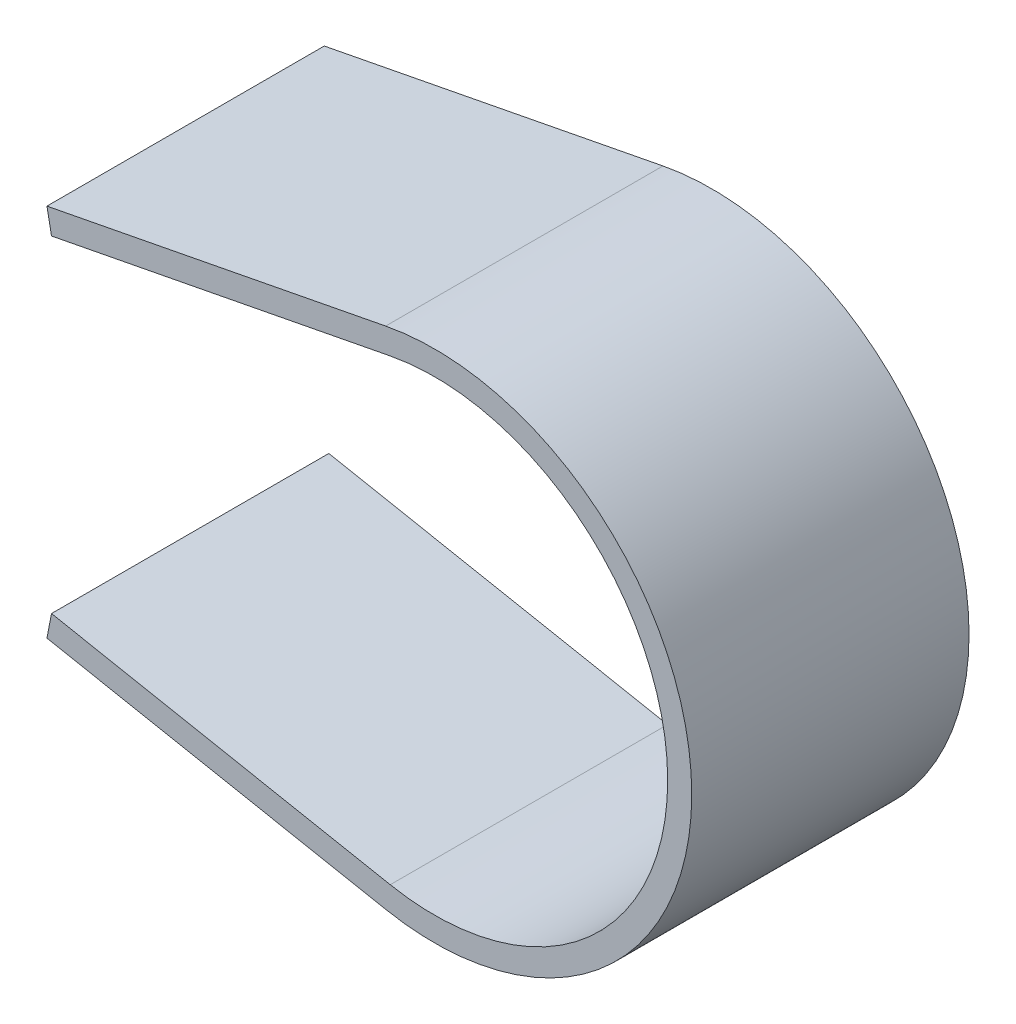
from build123d import *

# Parameters (mm, degrees)
BOSS_EXTRUDE1_DEPTH = 207.5


with BuildPart() as part:
    # Sketch1 → Boss-Extrude1 (new body)
    with BuildSketch(Plane.XY):
        with BuildLine():
            Line((-290, 140), (-36.538558432, 189.000486104))
            ThreePointArc((-36.538558432, 189.000486104), (192.5, 0), (-36.538558432, -189.000486104))
            Line((-36.538558432, -189.000486104), (-290, -140))
            Line((-290, -140), (-286.583407523, -122.327227273))
            Line((-286.583407523, -122.327227273), (-33.121965956, -171.327713378))
            ThreePointArc((-33.121965956, -171.327713378), (174.5, 0), (-33.121965956, 171.327713378))
            Line((-33.121965956, 171.327713378), (-286.583407523, 122.327227273))
            Line((-286.583407523, 122.327227273), (-290, 140))
        make_face()
    extrude(amount=BOSS_EXTRUDE1_DEPTH)


solid = part.part
